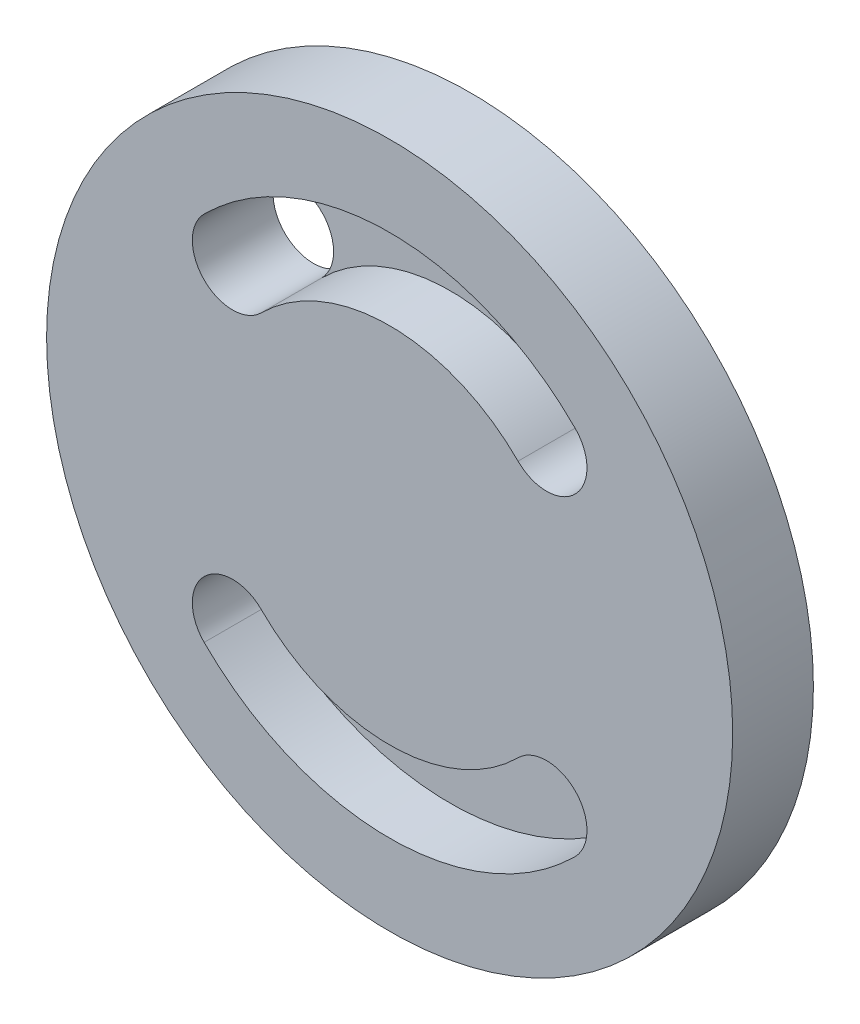
from build123d import *

# Parameters (mm, degrees)
SKETCH1_R           = 17
BOSS_EXTRUDE1_DEPTH = 4
CUT_EXTRUDE1_DEPTH  = 3
SKETCH3_R           = 2
CUT_EXTRUDE2_DEPTH  = 4
CUT_EXTRUDE3_DEPTH  = 3
SKETCH7_R           = 1.5
BOSS_EXTRUDE3_DEPTH = 2


with BuildPart() as part:
    # Sketch1 → Boss-Extrude1 (new body)
    with BuildSketch(Plane.XY):
        Circle(SKETCH1_R)
    extrude(amount=BOSS_EXTRUDE1_DEPTH)

    # Sketch2 → Cut-Extrude1 (cut)
    with BuildSketch(Plane.XY.offset(4)):
        with BuildLine():
            ThreePointArc((9.192388155, 9.192388155), (0, 13), (-9.192388155, 9.192388155))
            ThreePointArc((-9.192388155, 9.192388155), (-9.192388155, 6.363961031), (-6.363961031, 6.363961031))
            ThreePointArc((-6.363961031, 6.363961031), (0, 9), (6.363961031, 6.363961031))
            ThreePointArc((6.363961031, 6.363961031), (9.192388155, 6.363961031), (9.192388155, 9.192388155))
        make_face()
    extrude(amount=-CUT_EXTRUDE1_DEPTH, mode=Mode.SUBTRACT)

    # Sketch3 → Cut-Extrude2 (cut)
    with BuildSketch(Plane.XY.offset(4)):
        with Locations((7.778174593, 7.778174593)):
            Circle(SKETCH3_R)
        with Locations((-7.778174593, 7.778174593)):
            Circle(SKETCH3_R)
    extrude(amount=-CUT_EXTRUDE2_DEPTH, mode=Mode.SUBTRACT)

    # Sketch4 → Cut-Extrude3 (cut)
    with BuildSketch(Plane.XY.offset(4)):
        with BuildLine():
            ThreePointArc((-9.192388155, -9.192388155), (0, -13), (9.192388155, -9.192388155))
            ThreePointArc((9.192388155, -9.192388155), (9.192388155, -6.363961031), (6.363961031, -6.363961031))
            ThreePointArc((6.363961031, -6.363961031), (0, -9), (-6.363961031, -6.363961031))
            ThreePointArc((-6.363961031, -6.363961031), (-9.192388155, -6.363961031), (-9.192388155, -9.192388155))
        make_face()
    extrude(amount=-CUT_EXTRUDE3_DEPTH, mode=Mode.SUBTRACT)

    # Sketch7 → Boss-Extrude3 (add)
    with BuildSketch(Plane(origin=(0, 0, 0), x_dir=(-1, 0, 0), z_dir=(0, 0, -1))):
        with Locations(Location((11, 0, 0), (0, 0, 180))):
            Circle(SKETCH7_R)
        with Locations(Location((-11, 0, 0), (0, 0, 180))):
            Circle(SKETCH7_R)
    extrude(amount=BOSS_EXTRUDE3_DEPTH)


solid = part.part
